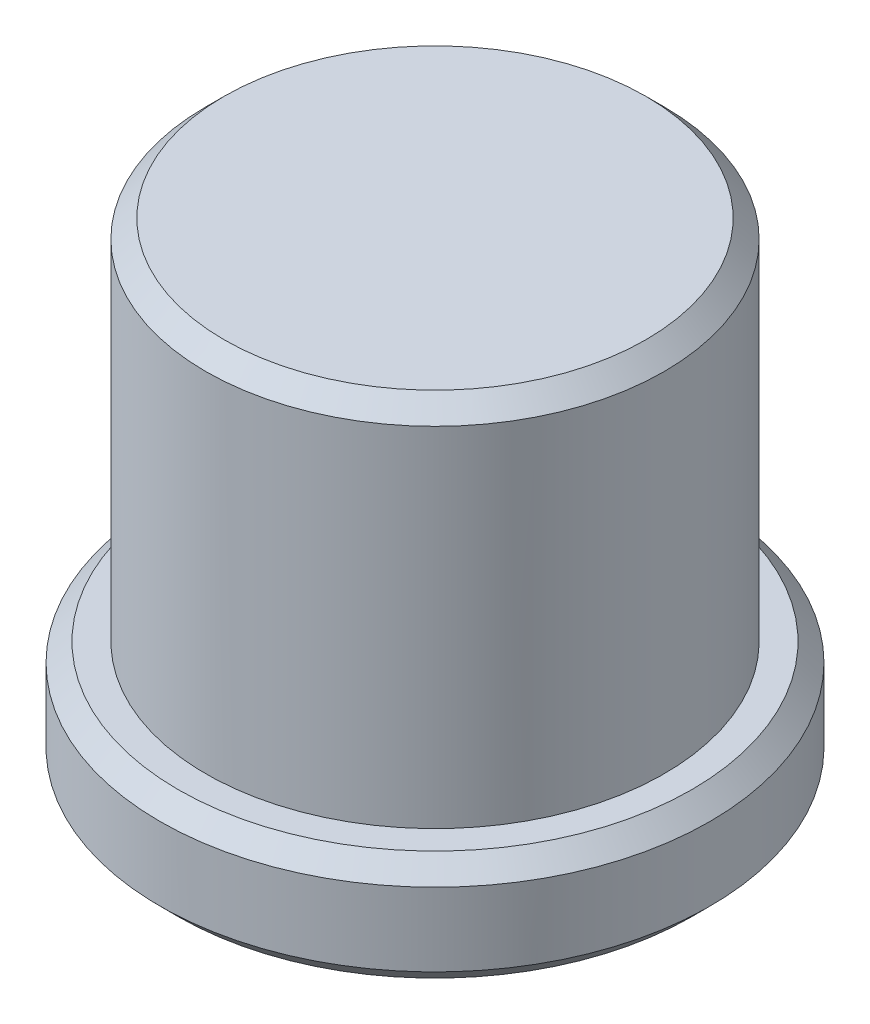
SolidWorks part; units mm, degrees
material "Q235B"
ref_plane "Front Plane" through (0, 0, 0) normal (0, 0, 1) x (1, 0, 0)
ref_plane "Top Plane" through (0, 0, 0) normal (0, 1, 0) x (1, 0, 0)
ref_plane "Right Plane" through (0, 0, 0) normal (1, 0, 0) x (0, 0, -1)
sketch "Sketch1" plane through (0, 0, 0) normal (1, 0, 0) x (0, 0, -1)
  line L0 (0, 0) -> (0, 13) construction
  line L1 (0, 13) -> (6.25, 13)
  line L2 (6.25, 13) -> (6.25, 3)
  line L3 (6.25, 3) -> (7.5, 3)
  line L4 (7.5, 3) -> (7.5, 0)
  line L5 (7.5, 0) -> (0, 0)
  line L6 (0, 0) -> (0, 13)
  dimension "D1" = 12.5
  dimension "D2" = 15
  dimension "D3" = 3
  dimension "D4" = 10
revolve "Revolve1" add sketch "Sketch1" angle 360 about L0
chamfer "Chamfer1" distance 0.5 angle 45 3 edges at (0, 0, -7.5) (0, 3, -7.5) (0, 13, -6.25)
